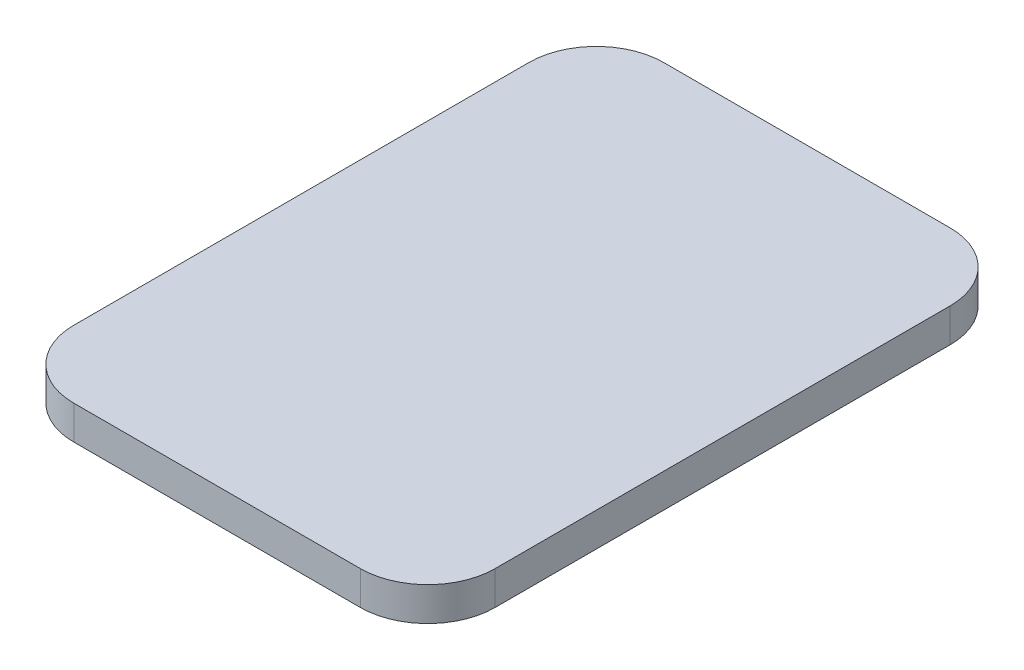
SolidWorks part; units mm, degrees
ref_plane "Plan de face" through (0, 0, 0) normal (0, 0, 1) x (1, 0, 0)
ref_plane "Plan de dessus" through (0, 0, 0) normal (0, 1, 0) x (1, 0, 0)
ref_plane "Plan de droite" through (0, 0, 0) normal (1, 0, 0) x (0, 0, -1)
sketch "Sketch1" plane through (0, 0, 0) normal (0, 1, 0) x (1, 0, 0)
  line L0 (8.5, 17.5) -> (-8.5, 17.5)
  line L1 (-12.5, 13.5) -> (-12.5, -13.5)
  line L2 (-8.5, -17.5) -> (8.5, -17.5)
  line L3 (12.5, -13.5) -> (12.5, 13.5)
  arc A0 (12.5, 13.5) -> (8.5, 17.5) centre (8.5, 13.5) ccw
  arc A1 (-8.5, 17.5) -> (-12.5, 13.5) centre (-8.5, 13.5) ccw
  arc A2 (-12.5, -13.5) -> (-8.5, -17.5) centre (-8.5, -13.5) ccw
  arc A3 (8.5, -17.5) -> (12.5, -13.5) centre (8.5, -13.5) ccw
extrude "Boss.-Extru.1" add sketch "Sketch1" along normal blind 2
